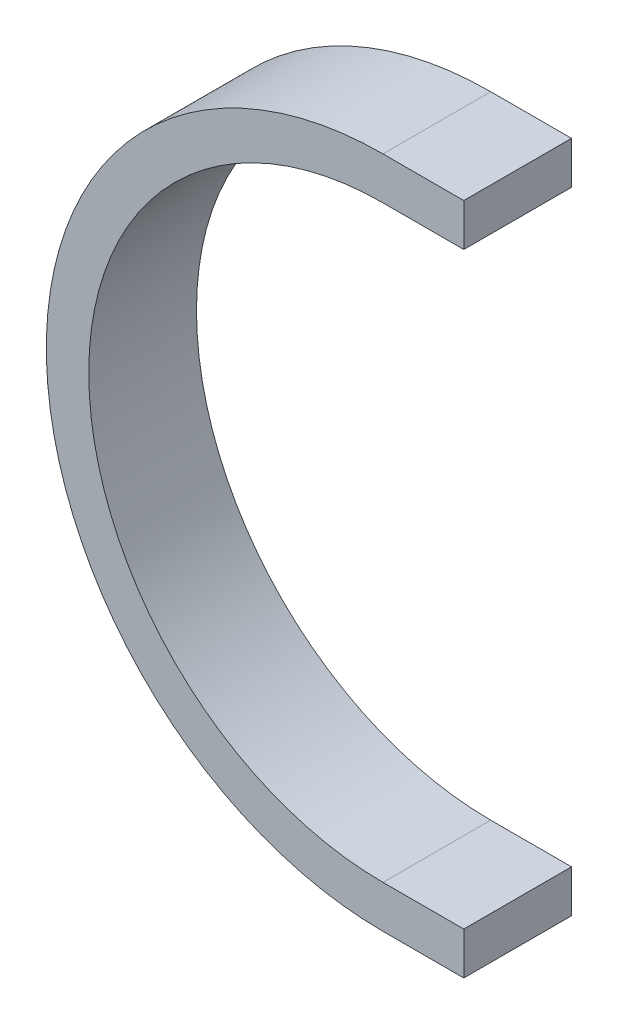
from build123d import *

# Parameters (mm, degrees)
BOSS_EXTRUDE1_DEPTH = 12.7


with BuildPart() as part:
    # Sketch1 → Boss-Extrude1 (new, symmetric)
    with BuildSketch(Plane.XY):
        with BuildLine():
            Line((0, 79.375), (19.05, 79.375))
            Line((19.05, 79.375), (19.05, 69.375))
            Line((19.05, 69.375), (0, 69.375))
            ThreePointArc((0, 69.375), (-69.375, 0), (0, -69.375))
            Line((0, -69.375), (19.05, -69.375))
            Line((19.05, -69.375), (19.05, -79.375))
            Line((19.05, -79.375), (0, -79.375))
            ThreePointArc((0, -79.375), (-79.375, 0), (0, 79.375))
        make_face()
    extrude(amount=BOSS_EXTRUDE1_DEPTH, both=True)


solid = part.part
